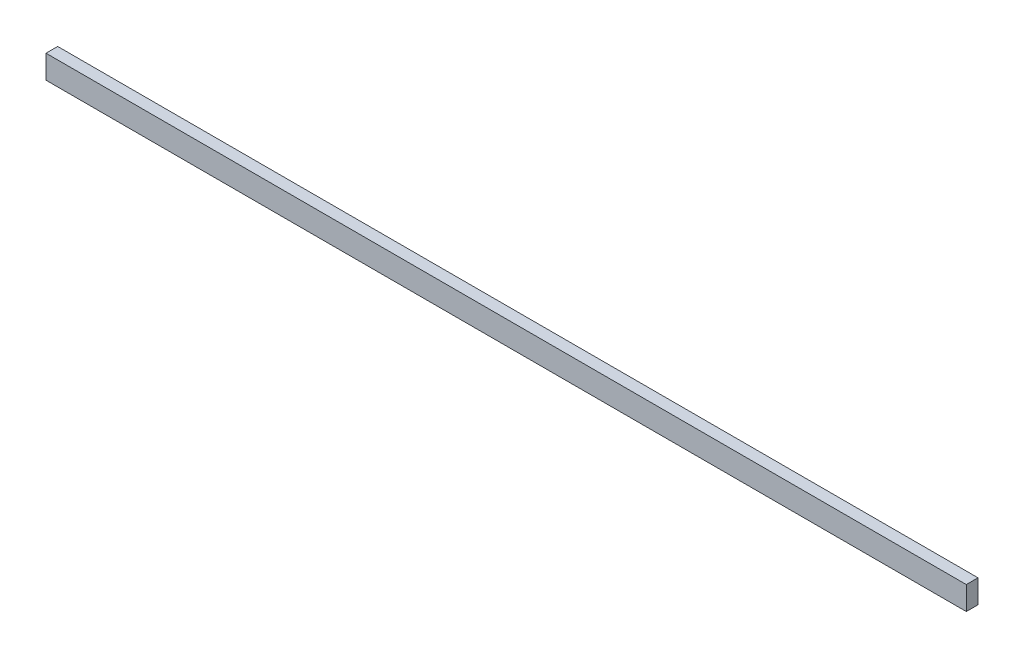
from build123d import *

# Parameters (mm, degrees)
SKETCH_1_W      = 1180
SKETCH_1_H      = 15
EXTRUDE_1_DEPTH = 15


with BuildPart() as part:
    # 草图1 → 凸台-拉伸1 (new, symmetric)
    with BuildSketch(Plane(origin=(0, 0, 0), x_dir=(1, 0, 0), z_dir=(0, 1, 0))):
        Rectangle(SKETCH_1_W, SKETCH_1_H)
    extrude(amount=EXTRUDE_1_DEPTH, both=True)


solid = part.part
